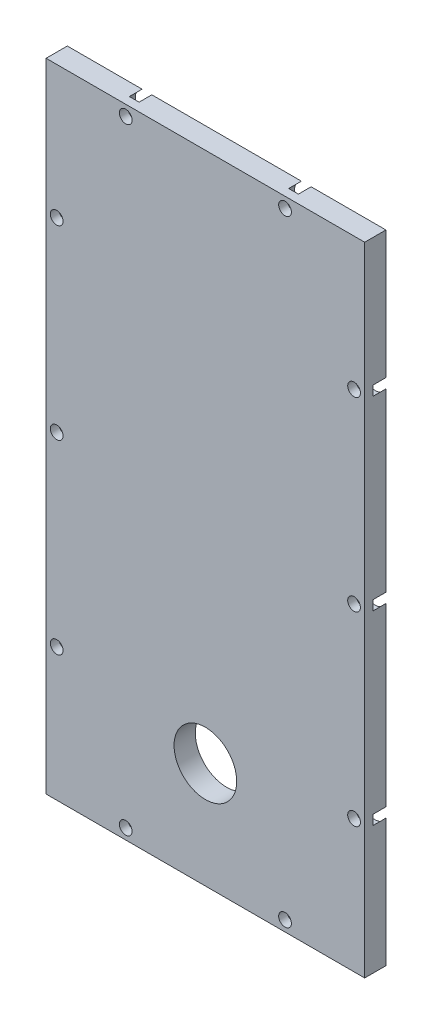
from build123d import *

# Parameters (mm, degrees)
SKETCH_1_W                   = 60
SKETCH_1_H                   = 120
EXTRUDE_1_DEPTH              = 2
HOLE_WIZARD_M2_1_D           = 2.4
HOLE_WIZARD_M2_1_CBORE_D     = 4.4
HOLE_WIZARD_M2_1_CBORE_DEPTH = 2.4
SKETCH_7_R                   = 5.9
CUT_EXTRUDE_2_DEPTH          = 68.201190466


with BuildPart() as part:
    # 草图1 → 凸台-拉伸1 (new, symmetric)
    with BuildSketch(Plane.XY):
        Rectangle(SKETCH_1_W, SKETCH_1_H)
    extrude(amount=EXTRUDE_1_DEPTH, both=True)

    # M2 六角凹头螺钉的柱形沉头孔1 (through all)
    with Locations(Plane(origin=(0, 0, -2), x_dir=(-1, 0, 0), z_dir=(0, 0, -1))):
        with Locations((-15, -58), (-28, 0), (28, 0), (-15, 58), (15, 58), (-28, 35), (28, 35), (-28, -35), (28, -35), (15, -58)):
            CounterBoreHole(HOLE_WIZARD_M2_1_D / 2, HOLE_WIZARD_M2_1_CBORE_D / 2, HOLE_WIZARD_M2_1_CBORE_DEPTH)

    # 草图7 → 切除-拉伸2 (cut, through all)
    with BuildSketch(Plane(origin=(0, 0, -2), x_dir=(-1, 0, 0), z_dir=(0, 0, -1))):
        with Locations((0, -40)):
            Circle(SKETCH_7_R)
    extrude(amount=-CUT_EXTRUDE_2_DEPTH, mode=Mode.SUBTRACT)


solid = part.part
